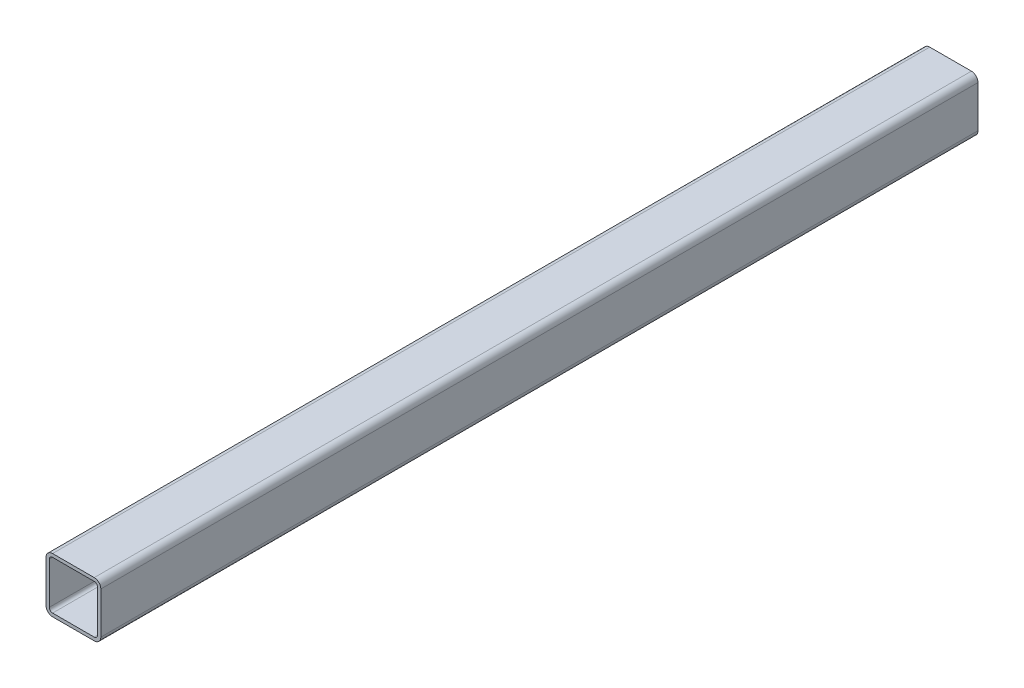
from build123d import *

# Parameters (mm, degrees)
GB_6728_1986_050_X_50_X_3_1_DEPTH = 800


with BuildPart() as part:
    # Sketch1 → Gb／6728-1986方形空心型钢 050 X 50 X 3(1) (new body)
    with BuildSketch(Plane.YX.offset(-400)):
        with BuildLine():
            Line((-19, -25), (19, -25))
            ThreePointArc((19, -25), (23.242640687, -23.242640687), (25, -19))
            Line((25, -19), (25, 19))
            ThreePointArc((25, 19), (23.242640687, 23.242640687), (19, 25))
            Line((19, 25), (-19, 25))
            ThreePointArc((-19, 25), (-23.242640687, 23.242640687), (-25, 19))
            Line((-25, 19), (-25, -19))
            ThreePointArc((-25, -19), (-23.242640687, -23.242640687), (-19, -25))
        make_face()
        with BuildLine():
            Line((-19, -22), (19, -22))
            ThreePointArc((19, -22), (21.121320344, -21.121320344), (22, -19))
            Line((22, -19), (22, 19))
            ThreePointArc((22, 19), (21.121320344, 21.121320344), (19, 22))
            Line((19, 22), (-19, 22))
            ThreePointArc((-19, 22), (-21.121320344, 21.121320344), (-22, 19))
            Line((-22, 19), (-22, -19))
            ThreePointArc((-22, -19), (-21.121320344, -21.121320344), (-19, -22))
        make_face(mode=Mode.SUBTRACT)
    extrude(amount=GB_6728_1986_050_X_50_X_3_1_DEPTH)


solid = part.part
